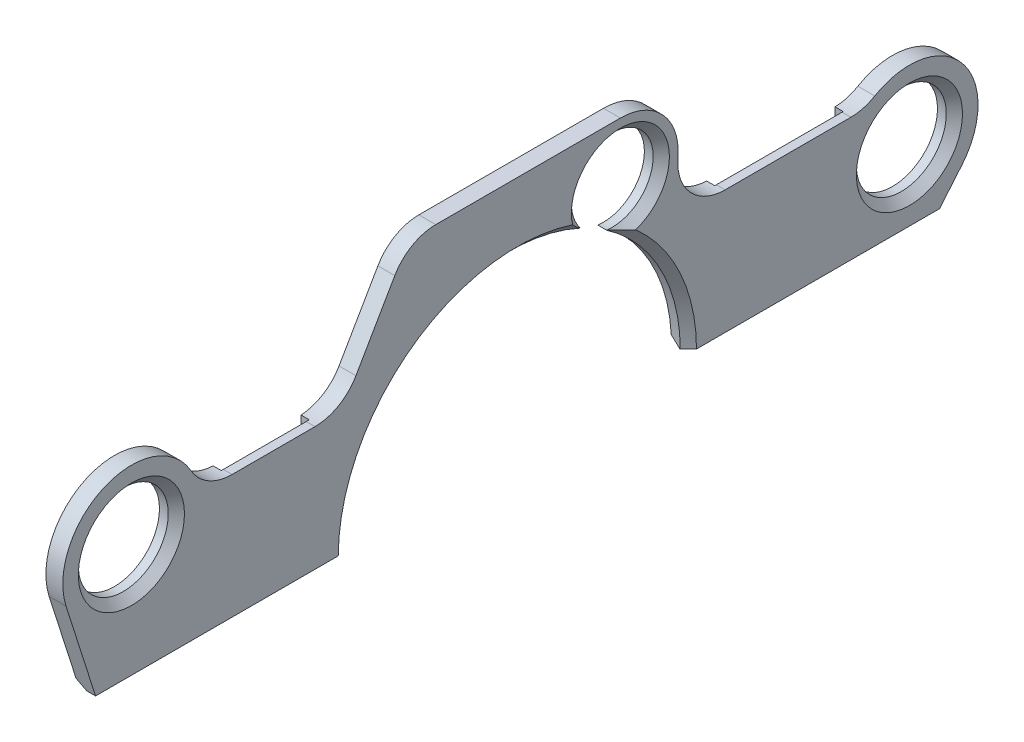
SolidWorks part; units mm, degrees
material "Q345B"
ref_plane "Front Plane" through (0, 0, 0) normal (0, 0, 1) x (1, 0, 0)
ref_plane "Top Plane" through (0, 0, 0) normal (0, 1, 0) x (1, 0, 0)
ref_plane "Right Plane" through (0, 0, 0) normal (1, 0, 0) x (0, 0, -1)
sketch "Sketch1" plane through (0, 0, 0) normal (1, 0, 0) x (0, 0, -1)
  line L0 (-1867.4529, 0) -> (418.1387, 0) construction
  line L1 (0, 339.4389) -> (0, -315.5279) construction
  line L2 (-161.1391, 353.5) -> (152.4, 353.5)
  line L3 (-161.1391, 353.5) -> (-259, 184)
  line L4 (-470.6145, 184) -> (-259, 184)
  line L6 (657.7535, 40.7571) -> (624.5612, 1.2)
  line L7 (307.2685, 184) -> (515.0519, 184)
  line L9 (-624, 1.2) -> (-667.6968, 138.1459)
  line L10 (624.5612, 1.2) -> (252.9972, 1.2)
  line L12 (-624, 1.2) -> (-252.9972, 1.2)
  arc A0 (237.5528, 260.3023) -> (307.2685, 184) centre (307.2685, 254) ccw
  arc A1 (252.9972, 1.2) -> (-252.9972, 1.2) centre (0, 0) ccw
  arc A2 (657.7535, 40.7571) -> (515.0519, 184) centre (580, 106) ccw
  arc A3 (-470.6145, 184) -> (-667.6968, 138.1459) centre (-571, 169) ccw
  arc A5 (237.5528, 260.3023) -> (152.4, 353.5) centre (152.4, 268) ccw
  dimension "D1" = 253
  dimension "D8" = 259
  dimension "D2" = 60
  dimension "D3" = 101.5
  dimension "D14" = 85.5
  dimension "D16" = 70
  dimension "D5" = 106
  dimension "D6" = 169
  dimension "D7" = 50
  dimension "D9" = 571
  dimension "D10" = 624
  dimension "D11" = 580
  dimension "D12" = 152.4
  dimension "D13" = 268
  dimension "D15" = 184
  dimension "D17" = 1.2
extrude "Boss-Extrude1" add sketch "Sketch1" along normal mid plane 25
sketch "Sketch2" plane through (0, 0, 0) normal (1, 0, 0) x (0, 0, -1)
  line L2 (-759.6656, 0) -> (783.6604, 0) construction
  line L3 (0, -128.1309) -> (0, 556.7634) construction
  circle A0 centre (152.4, 268) radius 60.5
  circle A1 centre (-571, 169) radius 66.5
  circle A2 centre (580, 106) radius 66.5
  dimension "D3" = 121
  dimension "D4" = 133
  dimension "D1" = 152.4
  dimension "D2" = 268
extrude "Cut-Extrude1" cut sketch "Sketch2" against normal through all both and the other way through all
fillet "Fillet1" radius 70 4 edges at (0, 184, -515.0519) (0, 353.5, 161.1391) (0, 184, 259) (0, 184, 470.6145)
chamfer "Chamfer1" distance 12 angle 45 5 edges at (12.5, 106, -646.5) (12.5, 213.2137, 136.1944) (12.5, 118.0184, -223.7871) (12.5, 320.5914, -182.3064) (12.5, 169, 504.5)
chamfer "Chamfer2" distance 12 angle 45 2 edges at (-12.5, 1.2, 438.4986) (-12.5, 1.2, -438.7792)
ref_plane "Plane1" through (0, 0, 360) normal (0, 0, 1) x (1, 0, 0)
ref_plane "Plane2" through (0, 0, -400) normal (0, 0, 1) x (1, 0, 0)
sketch "Sketch3" plane through (0, 0, 360) normal (0, 0, 1) x (1, 0, 0)
  line L0 (5.5, 190) -> (-12.5, 172)
  line L1 (-12.5, 172) -> (-12.5, 190)
  line L2 (-12.5, 190) -> (5.5, 190)
  line L4 (-12.5, 270.5) -> (-12.5, 138.1459) construction
  dimension "D1" = 45
  dimension "D2" = 172
  dimension "D3" = 190
extrude "Cut-Extrude2" cut sketch "Sketch3" against normal mid plane 130
sketch "Sketch4" plane through (0, 0, -400) normal (0, 0, 1) x (1, 0, 0)
  line L3 (-12.5, 172) -> (5.5, 190)
  line L4 (-12.5, 190) -> (-12.5, 172)
  line L5 (5.5, 190) -> (-12.5, 190)
  line L6 (-12.5, 172) -> (5.5, 190)
  line L7 (-12.5, 190) -> (-12.5, 172)
  line L8 (5.5, 190) -> (-12.5, 190)
  dimension "D1" = 0
extrude "Cut-Extrude3" cut sketch "Sketch4" against normal mid plane 190
